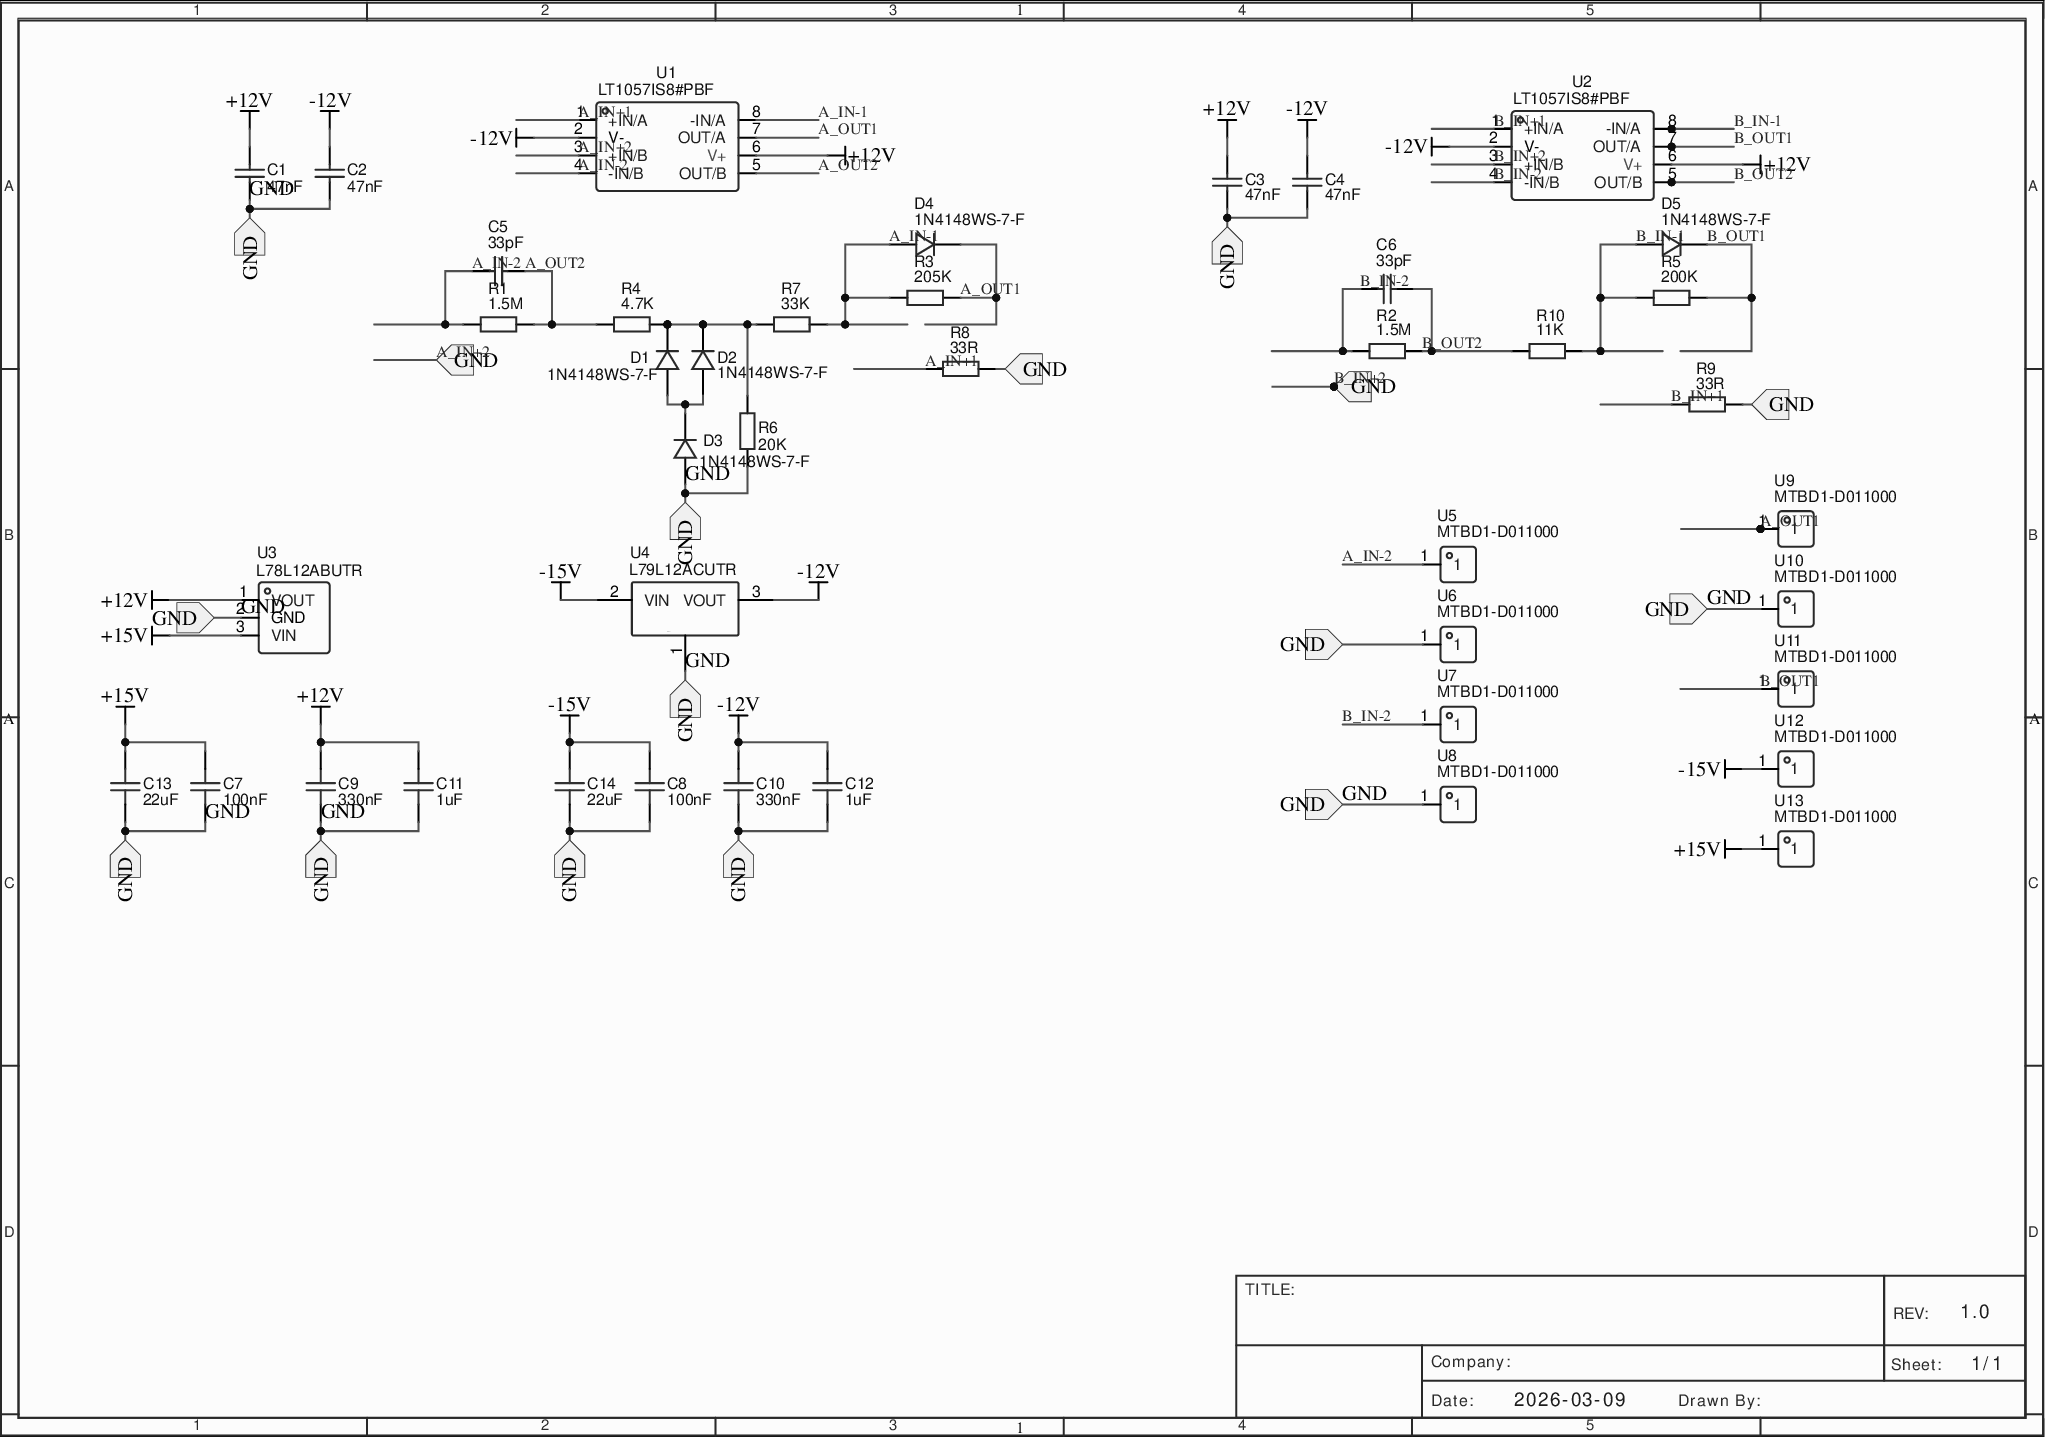
[diagram p0: MISC51764-3.schdoc]
# Altium project MISC51764-2.PrjPcb
1 sheet, 42 parts. Net scope: flat (ports and power ports of the same name join across sheets).
Board file: MISC51764.pcbdoc

## Sheet MISC51764-3.schdoc
size 292 x 205 mm; Name: MISC51764; @Project Name: MISC51764; REV: 1.0; Date: 2026-03-09; Sheet: 1/1; Manufacturer Part: ?

### Parts
C1  47nF  [C0603]
C2  47nF  [C0603]
C3  47nF  [C0603]
C4  47nF  [C0603]
C5  33pF  [C0603]
C6  33pF  [C0603]
C7  100nF  [C0603]
C8  100nF  [C0603]
C9  330nF  [C0603]
C10  330nF  [C0603]
C11  1uF  [C0603]
C12  1uF  [C0603]
C13  22uF  [C1210]
C14  22uF  [C1210]
D1  1N4148WS-7-F  [SOD-323_L1.8-W1.3-LS2.5-RD]
D2  1N4148WS-7-F  [SOD-323_L1.8-W1.3-LS2.5-RD]
D3  1N4148WS-7-F  [SOD-323_L1.8-W1.3-LS2.5-RD]
D4  1N4148WS-7-F  [SOD-323_L1.8-W1.3-LS2.5-RD]
D5  1N4148WS-7-F  [SOD-323_L1.8-W1.3-LS2.5-RD]
R1  1.5M  [R0603]
R2  1.5M  [R0603]
R3  205K  [R0603]
R4  4.7K  [R0603]
R5  200K  [R0603]
R6  20K  [R0603]
R7  33K  [R0603]
R8  33R  [R0603]
R9  33R  [R0603]
R10  11K  [R0603]
U1  LT1057IS8#PBF  [SOIC-8_L5.0-W4.0-P1.27-LS6.0-BL]
U2  LT1057IS8#PBF  [SOIC-8_L5.0-W4.0-P1.27-LS6.0-BL]
U3  L78L12ABUTR  [SOT-89-3_L4.5-W2.5-P1.50-LS4.2-BR]
U4  L79L12ACUTR  [SOT-89-3_L4.5-W2.5-P1.50-LS4.2-TL]
U5  MTBD1-D011000  [CR100]
U6  MTBD1-D011000  [CR100]
U7  MTBD1-D011000  [CR100]
U8  MTBD1-D011000  [CR100]
U9  MTBD1-D011000  [CR100]
U10  MTBD1-D011000  [CR100]
U11  MTBD1-D011000  [CR100]
U12  MTBD1-D011000  [CR100]
U13  MTBD1-D011000  [CR100]

### Ports
GND (in)

### Nets
+12V: C1.2 C3.2 C9.2 C11.2 U1.6(V+) U2.6(V+) U3.1(VOUT)
+15V: C7.2 C13.1 U3.3(VIN) U13.1
-12V: C2.2 C4.2 C10.2 C12.2 U1.2(V-) U2.2(V-) U4.3(VOUT)
-15V: C8.2 C14.1 U4.2(VIN) U12.1
A_IN+1: R8.1 U1.1(+IN/A)
A_IN+2: C1.1 C2.1 C3.1 C4.1 C7.1 C8.1 C9.1 C10.1 C11.1 C12.1 C13.2 C14.2 D3.2(A) R6.1 R8.2 R9.2 U1.3(+IN/B) U2.3(+IN/B) U3.2(GND) U4.1(GND) U6.1 U8.1 U10.1 ; port GND  [also labelled B_IN+2, GND]
A_IN-1: D4.2(A) R3.1 R7.2 U1.8(-IN/A)
A_IN-2: C5.1 R1.1 U1.4(-IN/B) U5.1
A_OUT1: D4.1(C) R3.2 U1.7(OUT/A) U9.1
A_OUT2: C5.2 R1.2 R4.1 U1.5(OUT/B)
B_IN+1: R9.1 U2.1(+IN/A)
B_IN-1: D5.2(A) R5.1 R10.2 U2.8(-IN/A)
B_IN-2: C6.1 R2.1 U2.4(-IN/B) U7.1
B_OUT1: D5.1(C) R5.2 U2.7(OUT/A) U11.1
B_OUT2: C6.2 R2.2 R10.1 U2.5(OUT/B)
NetD1_1: D1.1(C) D2.1(C) R4.2 R6.2 R7.1
NetD1_2: D1.2(A) D2.2(A) D3.1(C)

### Notes on the sheet
- 1
- 2
- 3
- 4
- 5
- A
- B
- C
- D
- TITLE:
- Company:
- Sheet:
- REV:
- 1.0
- 1/1
- Date:
- 2026-03-09
- Drawn By:

### Library data of the parts
C1 = CL10B473KB8NNNC: Manufacturer: SAMSUNG(三星); Convert to PCB: yes; UniqueId: gge9c184f7c30402505; OriginModelName: C0603_L1.6-W0.8-H0.8; ModelTransform: 62.992,31.496,0,0,0,0,0,0,0; Device: CL10B473KB8NNNC; Supplier: LCSC; Manufacturer Part: CL10B473KB8NNNC; Supplier Part: C1622; JLCPCB Part Class: Basic Part; Add into BOM: yes; SymbolName: 47nF; FootprintName: C0603
C2 = CL10B473KB8NNNC: Manufacturer: SAMSUNG(三星); Convert to PCB: yes; UniqueId: gge7dfa9a9d6c6b904b; OriginModelName: C0603_L1.6-W0.8-H0.8; ModelTransform: 62.992,31.496,0,0,0,0,0,0,0; Device: CL10B473KB8NNNC; Supplier: LCSC; Manufacturer Part: CL10B473KB8NNNC; Supplier Part: C1622; JLCPCB Part Class: Basic Part; Add into BOM: yes; SymbolName: 47nF; FootprintName: C0603
C3 = CL10B473KB8NNNC: Manufacturer: SAMSUNG(三星); Convert to PCB: yes; UniqueId: gge013fc20eec6c8c01; OriginModelName: C0603_L1.6-W0.8-H0.8; ModelTransform: 62.992,31.496,0,0,0,0,0,0,0; Device: CL10B473KB8NNNC; Supplier: LCSC; Manufacturer Part: CL10B473KB8NNNC; Supplier Part: C1622; JLCPCB Part Class: Basic Part; Add into BOM: yes; SymbolName: 47nF; FootprintName: C0603
C4 = CL10B473KB8NNNC: Manufacturer: SAMSUNG(三星); Convert to PCB: yes; UniqueId: gge944f94e5d51db243; OriginModelName: C0603_L1.6-W0.8-H0.8; ModelTransform: 62.992,31.496,0,0,0,0,0,0,0; Device: CL10B473KB8NNNC; Supplier: LCSC; Manufacturer Part: CL10B473KB8NNNC; Supplier Part: C1622; JLCPCB Part Class: Basic Part; Add into BOM: yes; SymbolName: 47nF; FootprintName: C0603
C5 = CL10C330JB8NNNC: Manufacturer: SAMSUNG(三星); Convert to PCB: yes; UniqueId: ggefcb32c91c6eb651c; OriginModelName: C0603_L1.6-W0.8-H0.8; ModelTransform: 62.992,31.496,0,0,0,0,0,0,0; Device: CL10C330JB8NNNC; Supplier: LCSC; Manufacturer Part: CL10C330JB8NNNC; Supplier Part: C1663; JLCPCB Part Class: Basic Part; Add into BOM: yes; SymbolName: 33pF; FootprintName: C0603
C6 = CL10C330JB8NNNC: Manufacturer: SAMSUNG(三星); Convert to PCB: yes; UniqueId: gge771bdc1ed411928b; OriginModelName: C0603_L1.6-W0.8-H0.8; ModelTransform: 62.992,31.496,0,0,0,0,0,0,0; Device: CL10C330JB8NNNC; Supplier: LCSC; Manufacturer Part: CL10C330JB8NNNC; Supplier Part: C1663; JLCPCB Part Class: Basic Part; Add into BOM: yes; SymbolName: 33pF; FootprintName: C0603
C7 = CGA0603X7R104K500JT: Manufacturer: HRE(芯声); Convert to PCB: yes; UniqueId: ggeb1a300cc2f1e9a25; OriginModelName: C0603_L1.6-W0.8-H0.8; ModelTransform: 62.992,31.496,0,0,0,0,0,0,0; Device: CGA0603X7R104K500JT; Supplier: LCSC; Supplier Part: C6119867; Manufacturer Part: CGA0603X7R104K500JT; JLCPCB Part Class: Extended Part; Add into BOM: yes; SymbolName: 100nF; FootprintName: C0603
C8 = CGA0603X7R104K500JT: Manufacturer: HRE(芯声); Convert to PCB: yes; UniqueId: ggece25ba8828fc93cc; OriginModelName: C0603_L1.6-W0.8-H0.8; ModelTransform: 62.992,31.496,0,0,0,0,0,0,0; Device: CGA0603X7R104K500JT; Supplier: LCSC; Supplier Part: C6119867; Manufacturer Part: CGA0603X7R104K500JT; JLCPCB Part Class: Extended Part; Add into BOM: yes; SymbolName: 100nF; FootprintName: C0603
C9 = FCC0603B334K500CT: Manufacturer: FOJAN(富捷); Convert to PCB: yes; UniqueId: gge26c64a3ce9fecbb4; OriginModelName: C0603_L1.6-W0.8-H0.8; ModelTransform: 62.992,31.496,0,0,0,0,0,0,0; Device: FCC0603B334K500CT; Supplier: LCSC; Supplier Part: C7419419; Manufacturer Part: FCC0603B334K500CT; JLCPCB Part Class: Extended Part; Add into BOM: yes; SymbolName: 330nF; FootprintName: C0603
C10 = FCC0603B334K500CT: Manufacturer: FOJAN(富捷); Convert to PCB: yes; UniqueId: ggeceb558a2caf91030; OriginModelName: C0603_L1.6-W0.8-H0.8; ModelTransform: 62.992,31.496,0,0,0,0,0,0,0; Device: FCC0603B334K500CT; Supplier: LCSC; Supplier Part: C7419419; Manufacturer Part: FCC0603B334K500CT; JLCPCB Part Class: Extended Part; Add into BOM: yes; SymbolName: 330nF; FootprintName: C0603
C11 = CGA0805X7R105K500MT: Manufacturer: HRE(芯声); Convert to PCB: yes; UniqueId: gge03546901c3460888; OriginModelName: C0603_L1.6-W0.8-H0.8; ModelTransform: 62.992,31.496,0,0,0,0,0,0,0; Device: CGA0805X7R105K500MT; Supplier: LCSC; Supplier Part: C6119929; Manufacturer Part: CGA0805X7R105K500MT; JLCPCB Part Class: Extended Part; Add into BOM: yes; SymbolName: 1uF; FootprintName: C0603
C12 = CGA0805X7R105K500MT: Manufacturer: HRE(芯声); Convert to PCB: yes; UniqueId: gge9b0487c796bd7391; OriginModelName: C0603_L1.6-W0.8-H0.8; ModelTransform: 62.992,31.496,0,0,0,0,0,0,0; Device: CGA0805X7R105K500MT; Supplier: LCSC; Supplier Part: C6119929; Manufacturer Part: CGA0805X7R105K500MT; JLCPCB Part Class: Extended Part; Add into BOM: yes; SymbolName: 1uF; FootprintName: C0603
C13 = CL32B226KAJNNNE: Manufacturer: SAMSUNG(三星); Convert to PCB: yes; UniqueId: gge3adf3cefc7429aa3; OriginModelName: C1210_L3.2-W2.5-H2.5; ModelTransform: 125.984,98.425,0,0,0,0,0,0.001,0; Device: CL32B226KAJNNNE; Supplier: LCSC; Supplier Part: C309062; Manufacturer Part: CL32B226KAJNNNE; JLCPCB Part Class: Extended Part; Add into BOM: yes; SymbolName: 22uF; FootprintName: C1210
C14 = CL32B226KAJNNNE: Manufacturer: SAMSUNG(三星); Convert to PCB: yes; UniqueId: gge9c5e47f948e52467; OriginModelName: C1210_L3.2-W2.5-H2.5; ModelTransform: 125.984,98.425,0,0,0,0,0,0.001,0; Device: CL32B226KAJNNNE; Supplier: LCSC; Supplier Part: C309062; Manufacturer Part: CL32B226KAJNNNE; JLCPCB Part Class: Extended Part; Add into BOM: yes; SymbolName: 22uF; FootprintName: C1210
D1 = 1N4148WS-7-F: Manufacturer: DIODES(美台); Convert to PCB: yes; UniqueId: gge930cf3e69b8057e6; ModelTransform: 104.3305,51.181,0,0,0,0,0,0,0; Device: 1N4148WS-7-F; Supplier: LCSC; Manufacturer Part: 1N4148WS-7-F; Supplier Part: C60580; JLCPCB Part Class: Extended Part; Add into BOM: yes; SymbolName: 1N4148WS-7-F; FootprintName: SOD-323_L1.8-W1.3-LS2.5-RD; OriginModelName: SOD-323_L1.8-W1.3-LS2.5-RD
D2 = 1N4148WS-7-F: Manufacturer: DIODES(美台); Convert to PCB: yes; UniqueId: gge611f15d2b5f3a7ed; ModelTransform: 104.3305,51.181,0,0,0,0,0,0,0; Device: 1N4148WS-7-F; Supplier: LCSC; Manufacturer Part: 1N4148WS-7-F; Supplier Part: C60580; JLCPCB Part Class: Extended Part; Add into BOM: yes; SymbolName: 1N4148WS-7-F; FootprintName: SOD-323_L1.8-W1.3-LS2.5-RD; OriginModelName: SOD-323_L1.8-W1.3-LS2.5-RD
D3 = 1N4148WS-7-F: Manufacturer: DIODES(美台); Convert to PCB: yes; UniqueId: ggeb8b107a3da1212ff; ModelTransform: 104.3305,51.181,0,0,0,0,0,0,0; Device: 1N4148WS-7-F; Supplier: LCSC; Manufacturer Part: 1N4148WS-7-F; Supplier Part: C60580; JLCPCB Part Class: Extended Part; Add into BOM: yes; SymbolName: 1N4148WS-7-F; FootprintName: SOD-323_L1.8-W1.3-LS2.5-RD; OriginModelName: SOD-323_L1.8-W1.3-LS2.5-RD
D4 = 1N4148WS-7-F: Manufacturer: DIODES(美台); Convert to PCB: yes; UniqueId: gge8f72676788cdbadf; ModelTransform: 104.3305,51.181,0,0,0,0,0,0,0; Device: 1N4148WS-7-F; Supplier: LCSC; Manufacturer Part: 1N4148WS-7-F; Supplier Part: C60580; JLCPCB Part Class: Extended Part; Add into BOM: yes; SymbolName: 1N4148WS-7-F; FootprintName: SOD-323_L1.8-W1.3-LS2.5-RD; OriginModelName: SOD-323_L1.8-W1.3-LS2.5-RD
D5 = 1N4148WS-7-F: Manufacturer: DIODES(美台); Convert to PCB: yes; UniqueId: gge89e0d268278955a4; ModelTransform: 104.3305,51.181,0,0,0,0,0,0,0; Device: 1N4148WS-7-F; Supplier: LCSC; Manufacturer Part: 1N4148WS-7-F; Supplier Part: C60580; JLCPCB Part Class: Extended Part; Add into BOM: yes; SymbolName: 1N4148WS-7-F; FootprintName: SOD-323_L1.8-W1.3-LS2.5-RD; OriginModelName: SOD-323_L1.8-W1.3-LS2.5-RD
R1 = 0603WAF1504T5E: Manufacturer: UNI-ROYAL(厚声); Convert to PCB: yes; UniqueId: gge275794aed69888ad; ModelTransform: 31.8897,63.7794,0,90,0,0,0,0,0; Device: 0603WAF1504T5E; Supplier: LCSC; Manufacturer Part: 0603WAF1504T5E; Supplier Part: C4172; JLCPCB Part Class: Extended Part; Add into BOM: yes; SymbolName: 1.5M; FootprintName: R0603; OriginModelName: R0603
R2 = 0603WAF1504T5E: Manufacturer: UNI-ROYAL(厚声); Convert to PCB: yes; UniqueId: gge62eca28fd27527f9; ModelTransform: 31.8897,63.7794,0,90,0,0,0,0,0; Device: 0603WAF1504T5E; Supplier: LCSC; Manufacturer Part: 0603WAF1504T5E; Supplier Part: C4172; JLCPCB Part Class: Extended Part; Add into BOM: yes; SymbolName: 1.5M; FootprintName: R0603; OriginModelName: R0603
R3 = 0603WAF1504T5E: Manufacturer: UNI-ROYAL(厚声); Convert to PCB: yes; UniqueId: gge38ffb8b7aac6ae1c; ModelTransform: 31.8897,63.7794,0,90,0,0,0,0,0; Device: 0603WAF1504T5E; Supplier: LCSC; Manufacturer Part: 0603WAF1504T5E; Supplier Part: C4172; JLCPCB Part Class: Extended Part; Add into BOM: yes; SymbolName: 205K; FootprintName: R0603; OriginModelName: R0603
R4 = 0603WAF1504T5E: Manufacturer: UNI-ROYAL(厚声); Convert to PCB: yes; UniqueId: gge06d0162e3aaf6f55; ModelTransform: 31.8897,63.7794,0,90,0,0,0,0,0; Device: 0603WAF1504T5E; Supplier: LCSC; Manufacturer Part: 0603WAF1504T5E; Supplier Part: C4172; JLCPCB Part Class: Extended Part; Add into BOM: yes; SymbolName: 4.7K; FootprintName: R0603; OriginModelName: R0603
R5 = 0603WAF1504T5E: Manufacturer: UNI-ROYAL(厚声); Convert to PCB: yes; UniqueId: gge24fdb472c9e249a5; ModelTransform: 31.8897,63.7794,0,90,0,0,0,0,0; Device: 0603WAF1504T5E; Supplier: LCSC; Manufacturer Part: 0603WAF1504T5E; Supplier Part: C4172; JLCPCB Part Class: Extended Part; Add into BOM: yes; SymbolName: 200K; FootprintName: R0603; OriginModelName: R0603
R6 = 0603WAF1504T5E: Manufacturer: UNI-ROYAL(厚声); Convert to PCB: yes; UniqueId: gge425e49353d1d2549; ModelTransform: 31.8897,63.7794,0,90,0,0,0,0,0; Device: 0603WAF1504T5E; Supplier: LCSC; Manufacturer Part: 0603WAF1504T5E; Supplier Part: C4172; JLCPCB Part Class: Extended Part; Add into BOM: yes; SymbolName: 20K; FootprintName: R0603; OriginModelName: R0603
R7 = 0603WAF1504T5E: Manufacturer: UNI-ROYAL(厚声); Convert to PCB: yes; UniqueId: gged7a0275a4f299522; ModelTransform: 31.8897,63.7794,0,90,0,0,0,0,0; Device: 0603WAF1504T5E; Supplier: LCSC; Manufacturer Part: 0603WAF1504T5E; Supplier Part: C4172; JLCPCB Part Class: Extended Part; Add into BOM: yes; SymbolName: 33K; FootprintName: R0603; OriginModelName: R0603
R8 = 0603WAF1504T5E: Manufacturer: UNI-ROYAL(厚声); Convert to PCB: yes; UniqueId: ggedd86cb9f7222bf07; ModelTransform: 31.8897,63.7794,0,90,0,0,0,0,0; Device: 0603WAF1504T5E; Supplier: LCSC; Manufacturer Part: 0603WAF1504T5E; Supplier Part: C4172; JLCPCB Part Class: Extended Part; Add into BOM: yes; SymbolName: 33R; FootprintName: R0603; OriginModelName: R0603
R9 = 0603WAF1504T5E: Manufacturer: UNI-ROYAL(厚声); Convert to PCB: yes; UniqueId: ggea5826b53fe23aaa4; ModelTransform: 31.8897,63.7794,0,90,0,0,0,0,0; Device: 0603WAF1504T5E; Supplier: LCSC; Manufacturer Part: 0603WAF1504T5E; Supplier Part: C4172; JLCPCB Part Class: Extended Part; Add into BOM: yes; SymbolName: 33R; FootprintName: R0603; OriginModelName: R0603
R10 = 0603WAF1504T5E: Manufacturer: UNI-ROYAL(厚声); Convert to PCB: yes; UniqueId: gge7c9623667e49f554; ModelTransform: 31.8897,63.7794,0,90,0,0,0,0,0; Device: 0603WAF1504T5E; Supplier: LCSC; Manufacturer Part: 0603WAF1504T5E; Supplier Part: C4172; JLCPCB Part Class: Extended Part; Add into BOM: yes; SymbolName: 11K; FootprintName: R0603; OriginModelName: R0603
U1 = LT1057IS8#PBF: Manufacturer: ADI(亚德诺); Convert to PCB: yes; UniqueId: ggede179d193d558ace; ModelTransform: 192.913,236.22,0,0,0,0,-0.001,0,0; Device: LT1057IS8#PBF; Supplier: LCSC; Supplier Part: C661570; Manufacturer Part: LT1057IS8#PBF; JLCPCB Part Class: Extended Part; Add into BOM: yes; SymbolName: LT1057IS8#PBF; FootprintName: SOIC-8_L5.0-W4.0-P1.27-LS6.0-BL; OriginModelName: SOIC-8_L5.0-W4.0-P1.27-LS6.0-BL
U2 = LT1057IS8#PBF: Manufacturer: ADI(亚德诺); Convert to PCB: yes; UniqueId: gge10e3e6eb1fb91831; ModelTransform: 192.913,236.22,0,0,0,0,-0.001,0,0; Device: LT1057IS8#PBF; Supplier: LCSC; Supplier Part: C661570; Manufacturer Part: LT1057IS8#PBF; JLCPCB Part Class: Extended Part; Add into BOM: yes; SymbolName: LT1057IS8#PBF; FootprintName: SOIC-8_L5.0-W4.0-P1.27-LS6.0-BL; OriginModelName: SOIC-8_L5.0-W4.0-P1.27-LS6.0-BL
U3 = L78L12ABUTR: Manufacturer: ST(意法半导体); Convert to PCB: yes; UniqueId: gge19d083384052ba2b; OriginModelName: SOT-89-3_L4.3-W2.5-H1.6-LS4.1-P1.50; ModelTransform: 161.417,169.291,0,0,0,0,12.744,0.004,0; Device: L78L12ABUTR; Supplier: LCSC; Supplier Part: C915681; Manufacturer Part: L78L12ABUTR; JLCPCB Part Class: Extended Part; Add into BOM: yes; SymbolName: L78L12ABUTR; FootprintName: SOT-89-3_L4.5-W2.5-P1.50-LS4.2-BR
U4 = L79L12ACUTR: Manufacturer: ST(意法半导体); Convert to PCB: yes; UniqueId: gge720bf4060678b6eb; OriginModelName: SOT-89-3_L4.3-W2.5-H1.6-LS4.1-P1.50; ModelTransform: 161.417,169.291,0,0,0,0,12.744,0.004,0; Device: L79L12ACUTR; Supplier: LCSC; Manufacturer Part: L79L12ACUTR; Supplier Part: C157399; JLCPCB Part Class: Extended Part; Add into BOM: yes; SymbolName: L79L12ACUTR; FootprintName: SOT-89-3_L4.5-W2.5-P1.50-LS4.2-TL
U5 = MTBD1-D011000: Manufacturer: MINTRON(明硕); Convert to PCB: yes; UniqueId: gged86c16d3e19e9c13; OriginModelName: CONN-TH_MTBD1-D011000; ModelTransform: 100.394,100,0,0,0,0,0,0,-118.11; Device: MTBD1-D011000; Supplier: LCSC; Supplier Part: C48983276; Manufacturer Part: MTBD1-D011000; JLCPCB Part Class: Extended Part; Add into BOM: yes; SymbolName: MTBD1-D011000; FootprintName: CR100
U6 = MTBD1-D011000: Manufacturer: MINTRON(明硕); Convert to PCB: yes; UniqueId: ggeb4f19fbd5e07dc59; OriginModelName: CONN-TH_MTBD1-D011000; ModelTransform: 100.394,100,0,0,0,0,0,0,-118.11; Device: MTBD1-D011000; Supplier: LCSC; Supplier Part: C48983276; Manufacturer Part: MTBD1-D011000; JLCPCB Part Class: Extended Part; Add into BOM: yes; SymbolName: MTBD1-D011000; FootprintName: CR100
U7 = MTBD1-D011000: Manufacturer: MINTRON(明硕); Convert to PCB: yes; UniqueId: gge9231cff1bd71fffb; OriginModelName: CONN-TH_MTBD1-D011000; ModelTransform: 100.394,100,0,0,0,0,0,0,-118.11; Device: MTBD1-D011000; Supplier: LCSC; Supplier Part: C48983276; Manufacturer Part: MTBD1-D011000; JLCPCB Part Class: Extended Part; Add into BOM: yes; SymbolName: MTBD1-D011000; FootprintName: CR100
U8 = MTBD1-D011000: Manufacturer: MINTRON(明硕); Convert to PCB: yes; UniqueId: gge7bf1ee9c5a71ae96; OriginModelName: CONN-TH_MTBD1-D011000; ModelTransform: 100.394,100,0,0,0,0,0,0,-118.11; Device: MTBD1-D011000; Supplier: LCSC; Supplier Part: C48983276; Manufacturer Part: MTBD1-D011000; JLCPCB Part Class: Extended Part; Add into BOM: yes; SymbolName: MTBD1-D011000; FootprintName: CR100
U9 = MTBD1-D011000: Manufacturer: MINTRON(明硕); Convert to PCB: yes; UniqueId: gge96b21cdb077c7bfb; OriginModelName: CONN-TH_MTBD1-D011000; ModelTransform: 100.394,100,0,0,0,0,0,0,-118.11; Device: MTBD1-D011000; Supplier: LCSC; Supplier Part: C48983276; Manufacturer Part: MTBD1-D011000; JLCPCB Part Class: Extended Part; Add into BOM: yes; SymbolName: MTBD1-D011000; FootprintName: CR100
U10 = MTBD1-D011000: Manufacturer: MINTRON(明硕); Convert to PCB: yes; UniqueId: gge01288fc0bb996d5a; OriginModelName: CONN-TH_MTBD1-D011000; ModelTransform: 100.394,100,0,0,0,0,0,0,-118.11; Device: MTBD1-D011000; Supplier: LCSC; Supplier Part: C48983276; Manufacturer Part: MTBD1-D011000; JLCPCB Part Class: Extended Part; Add into BOM: yes; SymbolName: MTBD1-D011000; FootprintName: CR100
U11 = MTBD1-D011000: Manufacturer: MINTRON(明硕); Convert to PCB: yes; UniqueId: ggeca0233f752f8c777; OriginModelName: CONN-TH_MTBD1-D011000; ModelTransform: 100.394,100,0,0,0,0,0,0,-118.11; Device: MTBD1-D011000; Supplier: LCSC; Supplier Part: C48983276; Manufacturer Part: MTBD1-D011000; JLCPCB Part Class: Extended Part; Add into BOM: yes; SymbolName: MTBD1-D011000; FootprintName: CR100
U12 = MTBD1-D011000: Manufacturer: MINTRON(明硕); Convert to PCB: yes; UniqueId: gge517e4af3480d1a88; OriginModelName: CONN-TH_MTBD1-D011000; ModelTransform: 100.394,100,0,0,0,0,0,0,-118.11; Device: MTBD1-D011000; Supplier: LCSC; Supplier Part: C48983276; Manufacturer Part: MTBD1-D011000; JLCPCB Part Class: Extended Part; Add into BOM: yes; SymbolName: MTBD1-D011000; FootprintName: CR100
U13 = MTBD1-D011000: Manufacturer: MINTRON(明硕); Convert to PCB: yes; UniqueId: ggeabc635ab583f020e; OriginModelName: CONN-TH_MTBD1-D011000; ModelTransform: 100.394,100,0,0,0,0,0,0,-118.11; Device: MTBD1-D011000; Supplier: LCSC; Supplier Part: C48983276; Manufacturer Part: MTBD1-D011000; JLCPCB Part Class: Extended Part; Add into BOM: yes; SymbolName: MTBD1-D011000; FootprintName: CR100